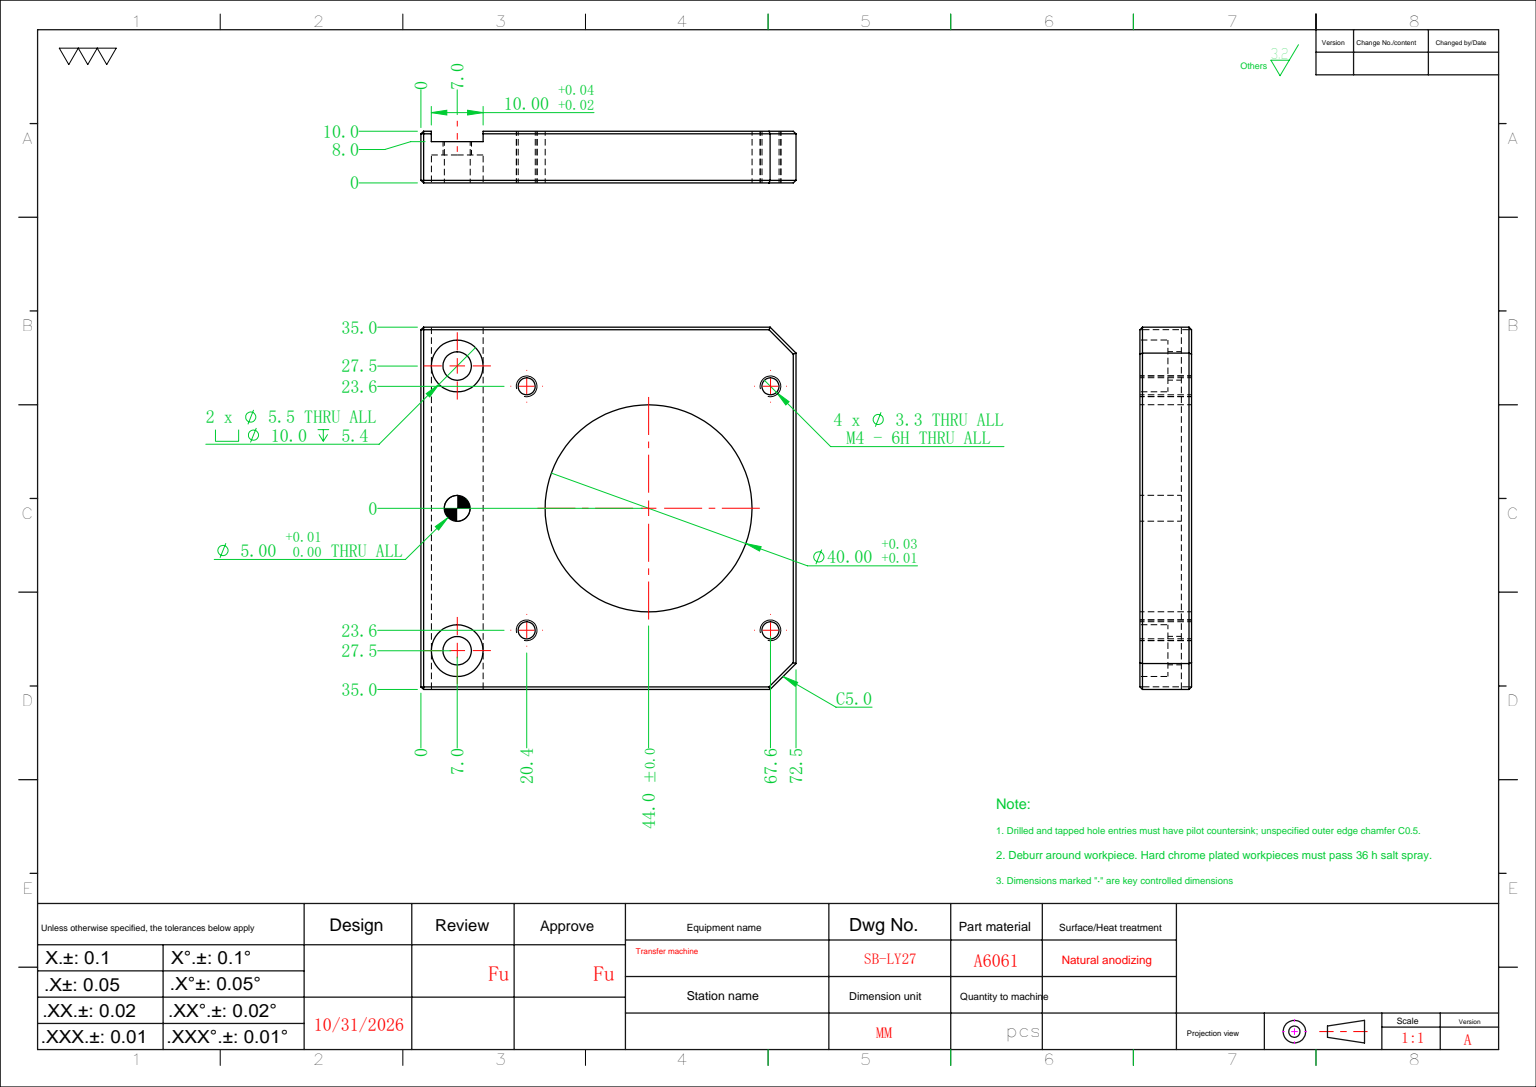
from build123d import *

# Parameters (mm, degrees)
SKETCH_1_W                   = 70
SKETCH_1_H                   = 72.5
EXTRUDE_1_DEPTH              = 10
SKETCH_2_W                   = 2
SKETCH_2_H                   = 10
CUT_EXTRUDE_1_DEPTH          = 80.461075377
HOLE_WIZARD_M5_1_D           = 5.5
HOLE_WIZARD_M5_1_CBORE_D     = 10
HOLE_WIZARD_M5_1_CBORE_DEPTH = 5.4
MM_1_D                       = 5
HOLE_WIZARD_M4_1_D           = 3.3
SKETCH_9_R                   = 20
CUT_EXTRUDE_2_DEPTH          = 52.37180647
CHAMFER_1_SIZE               = 5
CHAMFER_2_SIZE               = 0.5


with BuildPart() as part:
    # 草图1 → 凸台-拉伸1 (new body)
    with BuildSketch(Plane.XY):
        Rectangle(SKETCH_1_W, SKETCH_1_H)
    extrude(amount=EXTRUDE_1_DEPTH)

    # 草图2 → 切除-拉伸1 (cut, through all)
    with BuildSketch(Plane.ZY.offset(35)):
        with Locations((1, 29.25)):
            Rectangle(SKETCH_2_W, SKETCH_2_H)
    extrude(amount=-CUT_EXTRUDE_1_DEPTH, mode=Mode.SUBTRACT)

    # M5 六角凹头螺钉的柱形沉头孔1 (through all)
    with Locations(Plane.XY.offset(10)):
        with Locations((27.5, 29.25), (-27.5, 29.25)):
            CounterBoreHole(HOLE_WIZARD_M5_1_D / 2, HOLE_WIZARD_M5_1_CBORE_D / 2, HOLE_WIZARD_M5_1_CBORE_DEPTH)

    # 大小mm 暗销孔1 (through all)
    with Locations(Plane.XY.offset(10)):
        with Locations((0, 29.25)):
            Hole(MM_1_D / 2)

    # M4 螺纹孔1 (through all)
    with Locations(Plane.XY.offset(10)):
        with Locations((-23.57, 15.82), (-23.57, -31.32), (23.57, -31.32), (23.57, 15.82)):
            Hole(HOLE_WIZARD_M4_1_D / 2)

    # 草图9 → 切除-拉伸2 (cut, through all)
    with BuildSketch(Plane(origin=(0, 0, 0), x_dir=(-1, 0, 0), z_dir=(0, 0, -1))):
        with Locations((0, -7.75)):
            Circle(SKETCH_9_R)
    extrude(amount=-CUT_EXTRUDE_2_DEPTH, mode=Mode.SUBTRACT)

    # 倒角1
    chamfer_1_edges = [part.edges().sort_by_distance(p)[0] for p in [
        (35, -36.25, 5),
        (-35, -36.25, 5),
    ]]
    chamfer(chamfer_1_edges, length=CHAMFER_1_SIZE)

    # 倒角2
    chamfer_2_edges = [part.edges().sort_by_distance(p)[0] for p in [
        (35, 2.5, 10),
        (35, -3.5, 0),
        (0, -36.25, 0),
        (-32.5, -33.75, 0),
        (32.5, -33.75, 0),
        (0, -36.25, 10),
        (-32.5, -33.75, 10),
        (32.5, -33.75, 10),
        (-35, 2.5, 10),
        (35, 35.25, 0),
        (-35, -3.5, 0),
        (-35, 35.25, 0),
        (0, 36.25, 0),
        (-35, 36.25, 5),
        (35, 36.25, 5),
        (0, 36.25, 10),
    ]]
    chamfer(chamfer_2_edges, length=CHAMFER_2_SIZE)


solid = part.part
